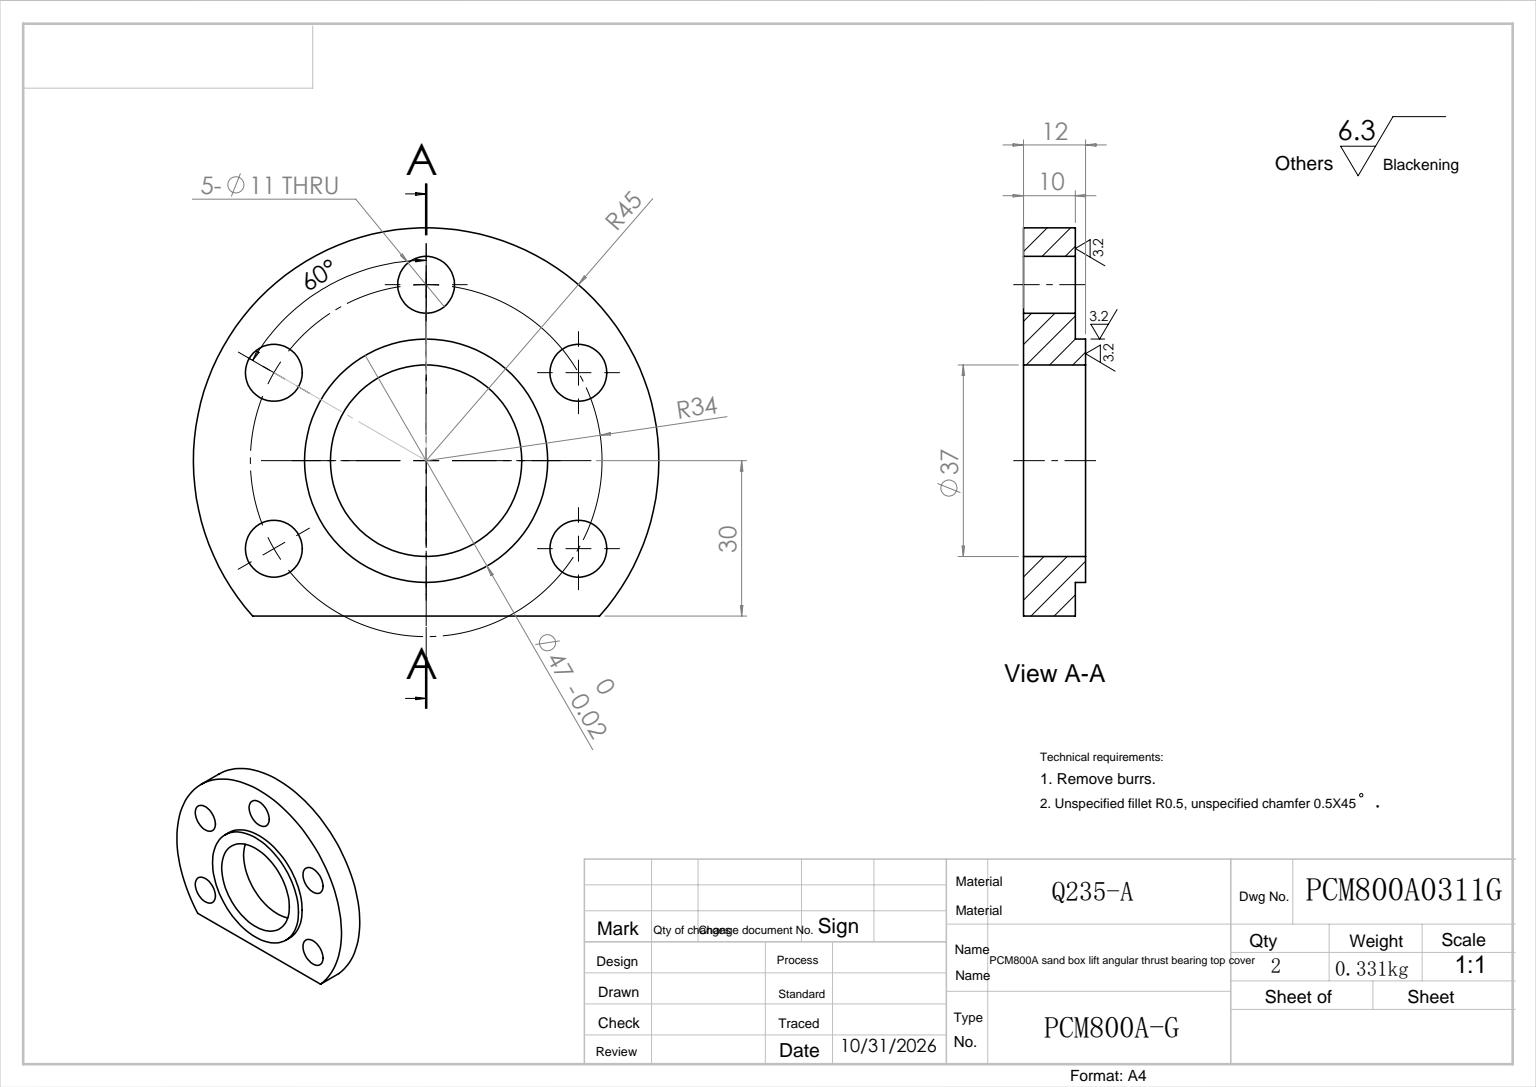
SolidWorks part; units mm, degrees
ref_plane "前视基准面" through (0, 0, 0) normal (0, 0, 1) x (1, 0, 0)
ref_plane "上视基准面" through (0, 0, 0) normal (0, 1, 0) x (1, 0, 0)
ref_plane "右视基准面" through (0, 0, 0) normal (1, 0, 0) x (0, 0, -1)
sketch "草图1" plane through (0, 0, 0) normal (0, 0, 1) x (1, 0, 0)
  circle A0 centre (0, 0) radius 45
  circle A1 centre (0, 0) radius 18.5
extrude "拉伸1" add sketch "草图1" along normal blind 10
sketch "草图2" plane through (0, 0, 10) normal (0, 0, 1) x (1, 0, 0)
  circle A0 centre (0, 0) radius 18.5
  circle A1 centre (0, 0) radius 23.5
extrude "拉伸2" add sketch "草图2" along normal blind 2
sketch "草图3" plane through (0, 0, 10) normal (0, 0, 1) x (1, 0, 0)
  line L0 (0, 0) -> (-38.3279, 22.1286) construction
  line L1 (0, 0) -> (36.5074, 21.0775) construction
  line L2 (0, 0) -> (0, 43.5532) construction
  line L3 (0, 0) -> (-49.1164, -28.3574) construction
  line L4 (0, 0) -> (54.0073, -31.1811) construction
  circle A0 centre (0, 0) radius 34 construction
  circle A1 centre (0, 34) radius 5.5
  circle A2 centre (-29.4449, 17) radius 5.5
  circle A3 centre (-29.4449, -17) radius 5.5
  circle A4 centre (29.4449, 17) radius 5.5
  circle A5 centre (29.4449, -17) radius 5.5
  dimension "D2" = 60
  dimension "D3" = 60
  dimension "D4" = 60
  dimension "D5" = 60
extrude "切除-拉伸1" cut sketch "草图3" against normal through all
sketch "草图4" plane through (0, 0, 10) normal (0, 0, 1) x (1, 0, 0)
  line L0 (-35.3887, -30) -> (35.3887, -30)
  arc A0 (-35.3887, -30) -> (35.3887, -30) centre (0, 0) ccw
  dimension "D1" = 30
extrude "切除-拉伸2" cut sketch "草图4" against normal through all
